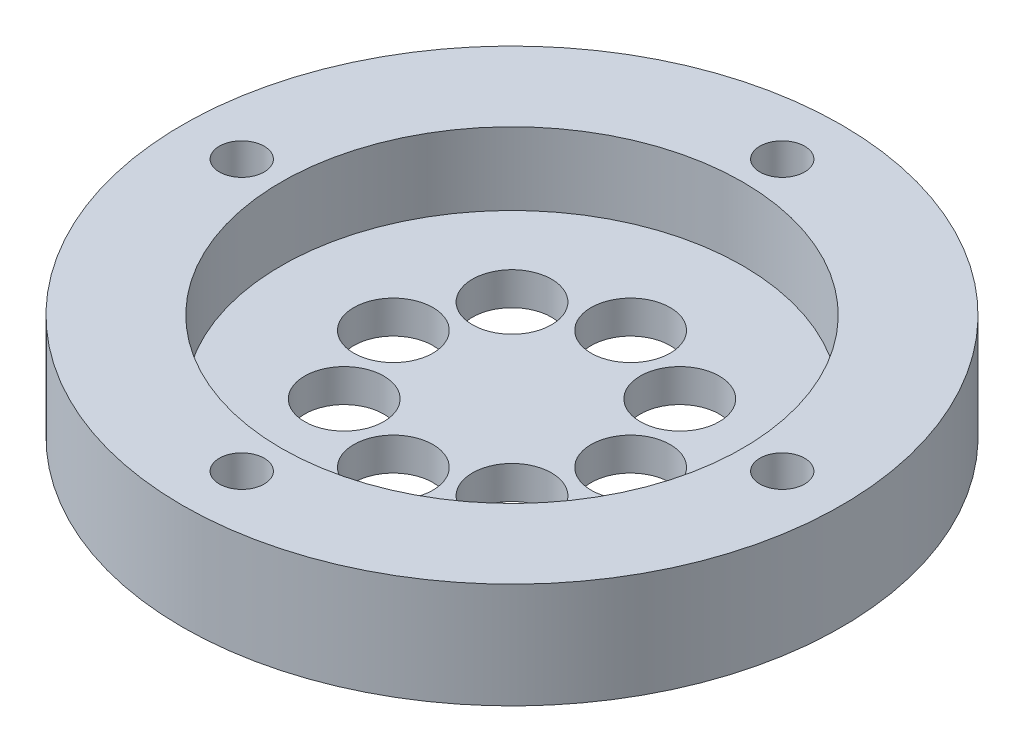
SolidWorks part; units mm, degrees
ref_plane "Front Plane" through (0, 0, 0) normal (0, 0, 1) x (1, 0, 0)
ref_plane "Top Plane" through (0, 0, 0) normal (0, 1, 0) x (1, 0, 0)
ref_plane "Right Plane" through (0, 0, 0) normal (1, 0, 0) x (0, 0, -1)
sketch "Sketch1" plane through (0, 0, 0) normal (0, 1, 0) x (1, 0, 0)
  circle A0 centre (0, 0) radius 25
  dimension "D1" = 50
extrude "Boss-Extrude1" add sketch "Sketch1" along normal blind 8
sketch "Sketch2" plane through (0, 8, 0) normal (0, 1, 0) x (1, 0, 0)
  circle A0 centre (0, 0) radius 17.5
  dimension "D1" = 35
extrude "Cut-Extrude1" cut sketch "Sketch2" against normal blind 5.5
sketch "Sketch3" plane through (0, 0, 0) normal (0, -1, 0) x (1, 0, 0)
  circle A0 centre (0, 0) radius 9 construction
  circle A1 centre (0, -9) radius 3
  circle A2 centre (-6.364, -6.364) radius 3
  circle A3 centre (-9, 0) radius 3
  circle A4 centre (-6.364, 6.364) radius 3
  circle A5 centre (0, 9) radius 3
  circle A6 centre (6.364, 6.364) radius 3
  circle A7 centre (9, 0) radius 3
  circle A8 centre (6.364, -6.364) radius 3
  point P21 (0, 0)
  dimension "D1" = 18
  dimension "D2" = 6
  dimension "D3" = 8
extrude "Cut-Extrude2" cut sketch "Sketch3" against normal blind 4
hole_wizard "CSK for M3 Flat Head Machine Screw1" positions "Sketch7" profile "Sketch8" countersink size "M3" standard "ANSI Metric" end condition through all
sketch "Sketch7" plane through (0, 0, 0) normal (0, -1, 0) x (-1, 0, 0)
  circle A0 centre (0, 0) radius 20.5 construction
  point P5 (0, 20.5)
  point P7 (-20.5, 0)
  point P9 (0, -20.5)
  point P11 (20.5, 0)
  dimension "D1" = 41
sketch "Sketch8" plane through (-20.5, 0, 0) normal (1, 0, 0) x (0, 0, -1)
  line L0 (0, 0) -> (0, 8)
  line L1 (0, 8) -> (1.7, 8)
  line L2 (1.7, 8) -> (1.7, 1.45)
  line L3 (1.7, 1.45) -> (3.15, 0)
  line L5 (3.15, 0) -> (0, 0)
  line L6 (-1.7, 1.45) -> (-3.15, 0) construction
  line L11 (0, -6.35) -> (0, 107.95) construction
  dimension "通孔孔直径" = 3.4
  dimension "通孔孔深度" = 8
  dimension "近端锥形沉头孔直径" = 6.3
  dimension "近端锥形沉头孔角度" = 90
